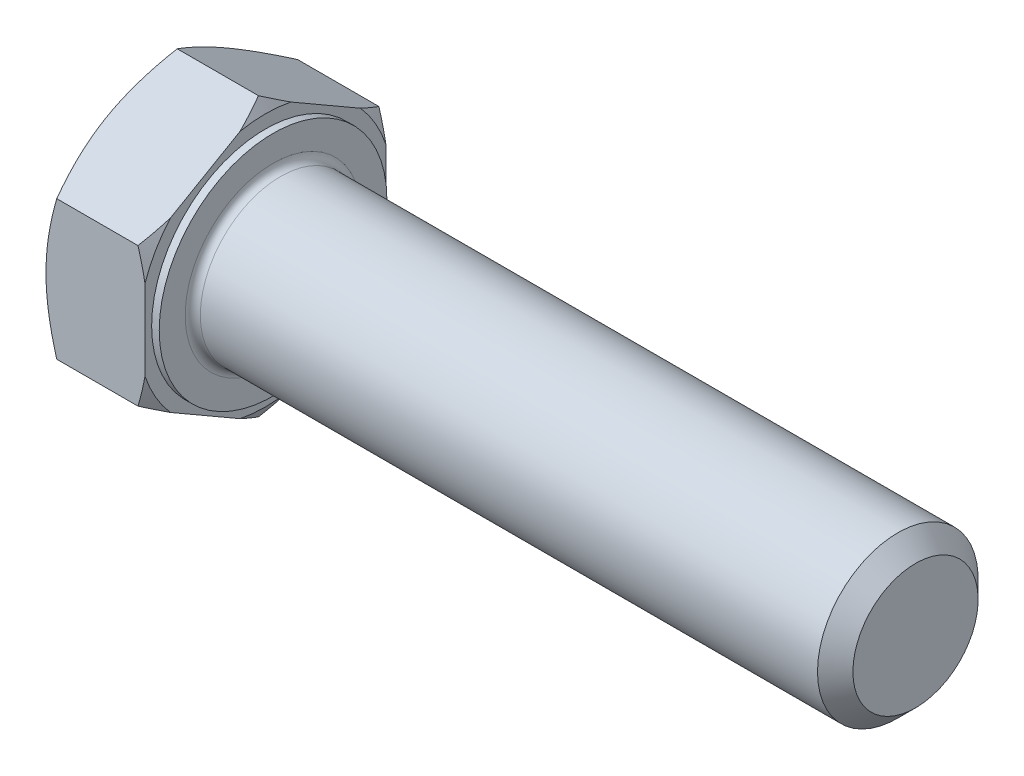
from build123d import *

# Parameters (mm, degrees)
BASE_EXTRUDE_DEPTH = 8.73125
SKETCH4_W          = 0.6
SKETCH4_H          = 11.998522628
CHAMFER_2_SIZE     = 1.4
FILLET_2_R         = 0.6


with BuildPart() as part:
    # Sketch1 → Base-Extrude (new body)
    with BuildSketch(Plane(origin=(0, 0, 0), x_dir=(0, 0, -1), z_dir=(1, 0, 0))):
        Polygon((9.525, 5.499261314), (9.525, -5.499261314), (0, -10.998522628), (-9.525, -5.499261314), (-9.525, 5.499261314), (0, 10.998522628), align=None)
    extrude(amount=BASE_EXTRUDE_DEPTH)

    # Sketch2 → Boss-Revolve1 (revolve)
    with BuildSketch(Plane.XY, mode=Mode.PRIVATE) as boss_revolve1_sk:
        Polygon((0, 0), (59.53125, 0), (59.53125, 5.55625), (59.53125, 6.35), (27.8072, 6.35), (0, 6.35), align=None)
    revolve(boss_revolve1_sk.sketch.rotate(Axis((0, 0, 0), (1, 0, 0)), 90), axis=Axis((0, 0, 0), (1, 0, 0)))

    # Sketch3 → Cut-Revolve1 (revolve, cut)
    with BuildSketch(Plane.XY, mode=Mode.PRIVATE) as cut_revolve1_sk:
        Polygon((0, 9), (4.040598923, 15.998522628), (4.040598923, 20.998522628), (-10, 20.998522628), (-10, 9), align=None)
    revolve(cut_revolve1_sk.sketch.rotate(Axis((0, 0, 0), (1, 0, 0)), 300.000000006), axis=Axis((0, 0, 0), (1, 0, 0)), mode=Mode.SUBTRACT)

    # Sketch5 → Cut-Revolve2 (revolve, cut)
    with BuildSketch(Plane.XY, mode=Mode.PRIVATE) as cut_revolve2_sk:
        Polygon((8.73125, 9), (4.690651077, 15.998522628), (4.690651077, 20.998522628), (14.690651077, 20.998522628), (14.690651077, 9), align=None)
    revolve(cut_revolve2_sk.sketch.rotate(Axis((0, 0, 0), (1, 0, 0)), 90), axis=Axis((0, 0, 0), (1, 0, 0)), mode=Mode.SUBTRACT)

    # Sketch4 → Cut-Revolve3 (revolve, cut)
    with BuildSketch(Plane.XY, mode=Mode.PRIVATE) as cut_revolve3_sk:
        with Locations((8.43125, 14.999261314)):
            Rectangle(SKETCH4_W, SKETCH4_H)
    revolve(cut_revolve3_sk.sketch.rotate(Axis((0, 0, 0), (1, 0, 0)), 90), axis=Axis((0, 0, 0), (1, 0, 0)), mode=Mode.SUBTRACT)

    # Chamfer 2
    chamfer_2_edges = [part.edges().sort_by_distance(p)[0] for p in [
        (59.53125, 0, -6.35),
    ]]
    chamfer(chamfer_2_edges, length=CHAMFER_2_SIZE)

    # Fillet 2
    fillet_2_edges = [part.edges().sort_by_distance(p)[0] for p in [
        (8.73125, 0, -6.35),
    ]]
    fillet(fillet_2_edges, radius=FILLET_2_R)


solid = part.part
